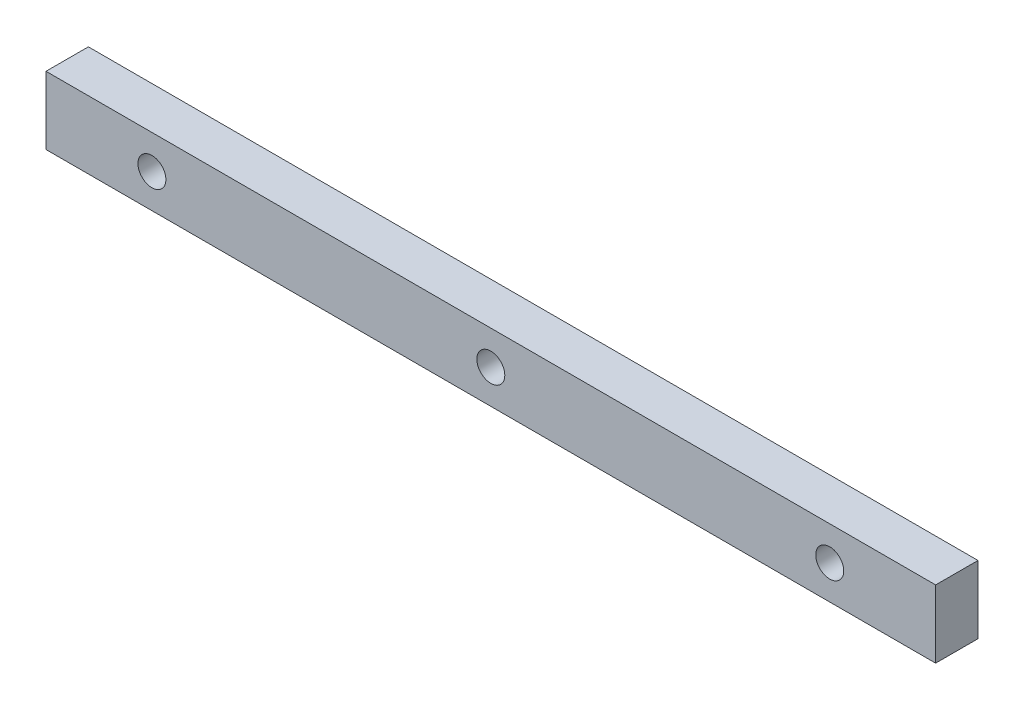
from build123d import *

# Parameters (mm, degrees)
SKETCH1_W           = 105
SKETCH1_H           = 8
BOSS_EXTRUDE1_DEPTH = 5
M4_TAPPED_HOLE2_D   = 3.3


with BuildPart() as part:
    # Sketch1 → Boss-Extrude1 (new body)
    with BuildSketch(Plane.XY):
        Rectangle(SKETCH1_W, SKETCH1_H)
    extrude(amount=BOSS_EXTRUDE1_DEPTH)

    # M4 Tapped Hole2 (through all)
    with Locations(Plane.XY.offset(5)):
        with Locations((-40, 0), (0, 0), (40, 0)):
            Hole(M4_TAPPED_HOLE2_D / 2)


solid = part.part
